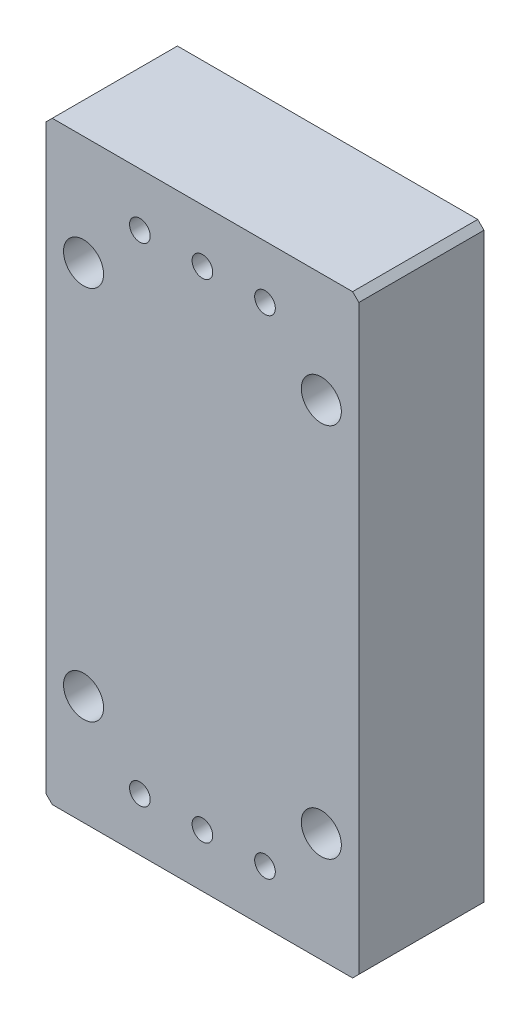
from build123d import *

# Parameters (mm, degrees)
SKETCH_1_W                   = 50
SKETCH_1_H                   = 95
EXTRUDE_1_DEPTH              = 20
HOLE_WIZARD_1_D              = 6.4
HOLE_WIZARD_1_CBORE_D        = 11
HOLE_WIZARD_1_CBORE_DEPTH    = 7
HOLE_WIZARD_M4_1_D           = 3.3
HOLE_WIZARD_M4_1_CSINK_D     = 4.05
HOLE_WIZARD_M4_1_CSINK_ANGLE = 90
CHAMFER_1_SIZE               = 1


with BuildPart() as part:
    # 草图1 → 凸台-拉伸1 (new body)
    with BuildSketch(Plane.XY):
        Rectangle(SKETCH_1_W, SKETCH_1_H)
    extrude(amount=EXTRUDE_1_DEPTH)

    # 打孔尺寸(%根据)内六角圆柱头螺钉的类型1 (through all)
    with Locations(Plane(origin=(0, 0, 0), x_dir=(-1, 0, 0), z_dir=(0, 0, -1))):
        with Locations((-19, 30), (-19, -30), (19, -30), (19, 30)):
            CounterBoreHole(HOLE_WIZARD_1_D / 2, HOLE_WIZARD_1_CBORE_D / 2, HOLE_WIZARD_1_CBORE_DEPTH)

    # M4 螺纹孔1 (through all)
    with Locations(Plane(origin=(0, 0, 0), x_dir=(-1, 0, 0), z_dir=(0, 0, -1))):
        with Locations((0, -39), (10, 39), (10, -39), (-10, -39), (-10, 39), (0, 39)):
            CounterSinkHole(HOLE_WIZARD_M4_1_D / 2, HOLE_WIZARD_M4_1_CSINK_D / 2, counter_sink_angle=HOLE_WIZARD_M4_1_CSINK_ANGLE)

    # 倒角1
    chamfer_1_edges = [part.edges().sort_by_distance(p)[0] for p in [
        (25, -47.5, 10),
        (-25, -47.5, 10),
        (-25, 47.5, 10),
        (25, 47.5, 10),
    ]]
    chamfer(chamfer_1_edges, length=CHAMFER_1_SIZE)


solid = part.part
